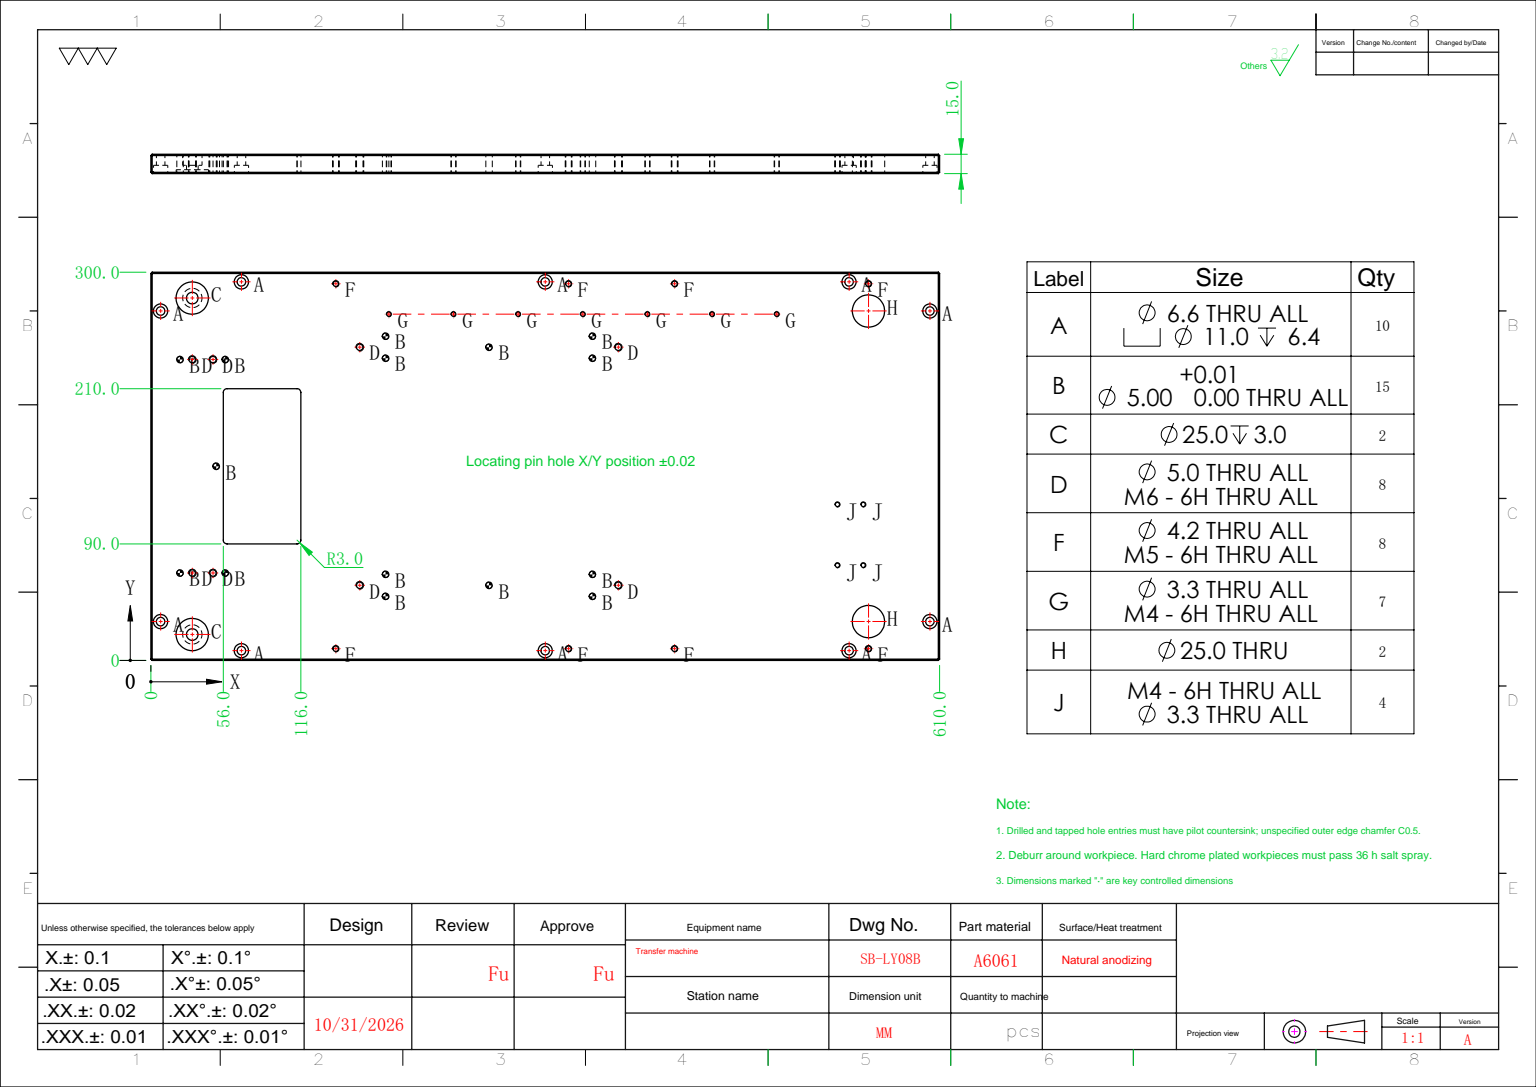
from build123d import *

# Parameters (mm, degrees)
SKETCH_1_W                     = 610
SKETCH_1_H                     = 300
EXTRUDE_1_DEPTH                = 15
SKETCH_25_R                    = 12.5
CUT_EXTRUDE_4_DEPTH            = 3
SKETCH_26_W                    = 60
SKETCH_26_H                    = 120
CUT_EXTRUDE_5_DEPTH            = 341.220516724
HOLE_WIZARD_M6_1_D             = 5
MM_1_D                         = 5
HOLE_WIZARD_M8_1_D             = 9
HOLE_WIZARD_M8_1_CBORE_D       = 15
HOLE_WIZARD_M8_1_CBORE_DEPTH   = 8.6
MM_0_D                         = 5
HOLE_WIZARD_M6_2_D             = 5
HOLE_WIZARD_M6_1_2_D           = 6.6
HOLE_WIZARD_M6_1_2_CBORE_D     = 11
HOLE_WIZARD_M6_1_2_CBORE_DEPTH = 6.4
HOLE_WIZARD_M4_1_D             = 3.3
PATTERN_LINEAR_1_COUNT         = 7
PATTERN_LINEAR_1_PITCH         = 50
HOLE_WIZARD_M5_1_D             = 4.2
SKETCH_46_R                    = 12.5
CUT_EXTRUDE_6_DEPTH            = 341.220516724
CHAMFER_1_SIZE                 = 1
HOLE_WIZARD_M4_2_D             = 3.3
FILLET_1_R                     = 3


with BuildPart() as part:
    # 草图1 → 凸台-拉伸1 (new body)
    with BuildSketch(Plane.XY):
        Rectangle(SKETCH_1_W, SKETCH_1_H)
    extrude(amount=EXTRUDE_1_DEPTH)

    # 草图25 → 切除-拉伸4 (cut)
    with BuildSketch(Plane.XY.offset(15)):
        with Locations((273, -130)):
            Circle(SKETCH_25_R)
        with Locations(Location((273, 130, 0), (0, 0, 180))):
            Circle(SKETCH_25_R)
    extrude(amount=-CUT_EXTRUDE_4_DEPTH, mode=Mode.SUBTRACT)

    # 草图26 → 切除-拉伸5 (cut, through all)
    with BuildSketch(Plane.XY.offset(15)):
        with Locations((219, 0)):
            Rectangle(SKETCH_26_W, SKETCH_26_H)
    extrude(amount=-CUT_EXTRUDE_5_DEPTH, mode=Mode.SUBTRACT)

    # Hole Wizard M6 _1 (through all)
    with Locations(Plane.XY.offset(15)):
        with Locations((143.500757595, -92), (-56.499242405, -92), (-56.499242405, 92), (143.500757595, 92)):
            Hole(HOLE_WIZARD_M6_1_D / 2)

    # 大小mm 暗销孔1 (through all)
    with Locations(Plane.XY.offset(15)):
        with Locations((123.500757595, -83.5), (123.500757595, -100.5), (43.500757595, -92), (-36.499242405, -100.5), (-36.499242405, -83.5), (-36.499242405, 83.5), (-36.499242405, 100.5), (123.500757595, 100.5), (123.500757595, 83.5), (43.500757595, 92)):
            Hole(MM_1_D / 2)

    # M8 六角凹头螺钉的柱形沉头孔1 (through all)
    with Locations(Plane(origin=(0, 0, 0), x_dir=(-1, 0, 0), z_dir=(0, 0, -1))):
        with Locations((-273, -130), (-273, 130)):
            CounterBoreHole(HOLE_WIZARD_M8_1_D / 2, HOLE_WIZARD_M8_1_CBORE_D / 2, HOLE_WIZARD_M8_1_CBORE_DEPTH)

    # 大小mm 暗销孔0 (through all)
    with Locations(Plane.XY.offset(15)):
        with Locations((282.5, -82.5), (282.5, 82.5), (247.5, 82.5), (247.5, -82.5), (254.5, 0)):
            Hole(MM_0_D / 2)

    # M6 螺纹孔2 (through all)
    with Locations(Plane.XY.offset(15)):
        with Locations((257, -82.5), (273, -82.5), (257, 82.5), (273, 82.5)):
            Hole(HOLE_WIZARD_M6_2_D / 2)

    # Hole Wizard M6 _1 2 (through all)
    with Locations(Plane.XY.offset(15)):
        with Locations((-297.5, -120), (-235, -142.5), (-235, 142.5), (-297.5, 120), (297.5, 120), (235, 142.5), (235, -142.5), (297.5, -120), (0, -142.5), (0, 142.5)):
            CounterBoreHole(HOLE_WIZARD_M6_1_2_D / 2, HOLE_WIZARD_M6_1_2_CBORE_D / 2, HOLE_WIZARD_M6_1_2_CBORE_DEPTH)

    # M4 螺纹孔1 (through all)
    with Locations(Plane.XY.offset(15)):
        with Locations((121.000757595, -117.5)):
            hole_wizard_m4_1 = Hole(HOLE_WIZARD_M4_1_D / 2)

    # 阵列(线性)1: M4 螺纹孔1 ×7
    with Locations(*[(-i * PATTERN_LINEAR_1_PITCH, 0, 0) for i in range(1, PATTERN_LINEAR_1_COUNT)]):
        add(hole_wizard_m4_1, mode=Mode.SUBTRACT)

    # M5 螺纹孔1 (through all)
    with Locations(Plane.XY.offset(15)):
        with Locations((-100, -141.0016), (-250, -141.0016), (-250, 141.0016), (-100, 141.0016), (-18, 141.0016), (162.000000007, 141.0016), (162.000000007, -141.0016), (-18, -141.0016)):
            Hole(HOLE_WIZARD_M5_1_D / 2)

    # 草图46 → 切除-拉伸6 (cut, through all)
    with BuildSketch(Plane.XY.offset(15)):
        with Locations((-250, -120)):
            Circle(SKETCH_46_R)
        with Locations(Location((-250, 120, 0), (0, 0, 180))):
            Circle(SKETCH_46_R)
    extrude(amount=-CUT_EXTRUDE_6_DEPTH, mode=Mode.SUBTRACT)

    # 倒角1
    chamfer_1_edges = [part.edges().sort_by_distance(p)[0] for p in [
        (-305, 0, 15),
        (0, -150, 15),
        (305, 0, 15),
        (0, -150, 0),
        (-305, 0, 0),
        (0, 150, 0),
        (305, 0, 0),
        (0, 150, 15),
        (305, -150, 7.5),
        (-305, -150, 7.5),
        (-305, 150, 7.5),
        (305, 150, 7.5),
    ]]
    chamfer(chamfer_1_edges, length=CHAMFER_1_SIZE)

    # M4 螺纹孔2 (through all)
    with Locations(Plane.XY.offset(15)):
        with Locations((-246, 76.5), (-226, 76.5), (-246, 29.5), (-226, 29.5)):
            Hole(HOLE_WIZARD_M4_2_D / 2)

    # 圆角1
    fillet_1_edges = [part.edges().sort_by_distance(p)[0] for p in [
        (189, -60, 7.5),
        (189, 60, 7.5),
        (249, 60, 7.5),
        (249, -60, 7.5),
    ]]
    fillet(fillet_1_edges, radius=FILLET_1_R)


solid = part.part
